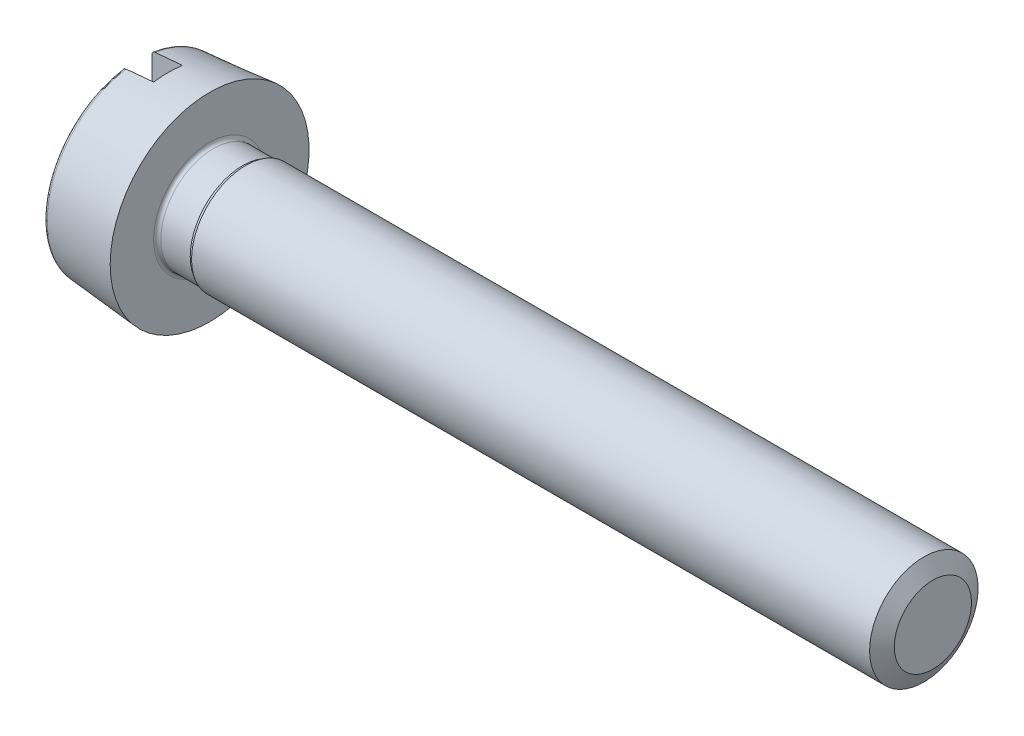
SolidWorks part; units mm, degrees
ref_plane "Front Plane" through (0, 0, 0) normal (0, 0, 1) x (1, 0, 0)
ref_plane "Top Plane" through (0, 0, 0) normal (0, 1, 0) x (1, 0, 0)
ref_plane "Right Plane" through (0, 0, 0) normal (1, 0, 0) x (0, 0, -1)
sketch "Dimensioned Sketch" plane through (0, 0, 0) normal (0, 0, 1) x (1, 0, 0)
  line L0 (0, 0) -> (22, 0) construction
  point P3 (0.85, 0)
  point P4 (1, 0)
  point P5 (3, 0)
  point P6 (5.5, 0)
  point P7 (0.8, 0)
  point P8 (9.1, 0)
  point P9 (9.85, 0)
  point P11 (21.5, 0)
  point P12 (21.9, 0)
  point P13 (2, 0)
  dimension "k" = 2
  dimension "t" = 0.85
  dimension "a" = 1
  dimension "d" = 3
  dimension "l" = 20
  dimension "dk" = 5.5
  dimension "n" = 0.8
  dimension "r" = 0.1
  dimension "p" = 0.5
  dimension "da" = 3.6
  dimension "w" = 0.75
sketch "Sketch1" plane through (0, 0, 0) normal (0, 0, 1) x (1, 0, 0)
  line L0 (0, 0) -> (22, 0) construction
  line L1 (0, 0) -> (0, 2.4834)
  line L2 (2, 2.75) -> (0.0913, 2.583)
  line L3 (2, 2.75) -> (2, 1.55)
  line L4 (2.1, 1.45) -> (2.9134, 1.45)
  line L5 (2.9134, 1.45) -> (3, 1.5)
  line L6 (3, 1.5) -> (22, 1.5)
  line L7 (22, 1.5) -> (22, 0)
  line L8 (0, 0) -> (22, 0)
  arc A0 (2.1, 1.45) -> (2, 1.55) centre (2.1, 1.55) cw
  arc A1 (0, 2.4834) -> (0.0913, 2.583) centre (0.1, 2.4834) cw
  dimension "r" = 0.1
  dimension "D10" = 0.1
  dimension "D1" = 2.9
  dimension "D2" = 85
  dimension "d" = 3
  dimension "a" = 1
  dimension "D8" = 30
  dimension "k" = 2
  dimension "dk" = 5.5
  dimension "l" = 20
revolve "Base-Revolve" add sketch "Sketch1" angle 360 about L0
cosmetic thread "Cosmetic Thread1" parameters "D2"=2.598
sketch "Sketch2" plane through (0, 0, 0) normal (-1, 0, 0) x (0, 0, 1)
  line L0 (0, 0) -> (0, -1.8809) construction
  line L3 (0.4, 2.7208) -> (0.4, -2.7208)
  line L5 (-0.4, 2.7208) -> (-0.4, -2.7208)
  circle A1 centre (0, 0) radius 2.75 construction
  arc A2 (0.4, 2.7208) -> (-0.4, 2.7208) centre (0, 0) ccw
  arc A3 (-0.4, -2.7208) -> (0.4, -2.7208) centre (0, 0) ccw
  dimension "n" = 0.8
extrude "Cut-Extrude1" cut sketch "Sketch2" against normal blind 0.85
sketch "Sketch3" plane through (0, 0, 0) normal (0, 1, 0) x (1, 0, 0)
  line L0 (21.75, 1.5) -> (22.25, 1.5)
  line L2 (22.25, 1.5) -> (22, 1.067)
  line L3 (22, 1.067) -> (21.75, 1.5)
  line L4 (22, -1.6037) -> (22, 0) construction
  line L10 (22, -1.5) -> (22, 1.5) construction
  line L11 (0, 0) -> (7.2232, 0) construction
  dimension "D2" = 0.433
  dimension "D3" = 1.5
revolve "Cut-Revolve1" cut sketch "Sketch3" angle 360 about L11
pattern_linear "LPattern1" [suppressed] count 39 along (1, 0, 0)
